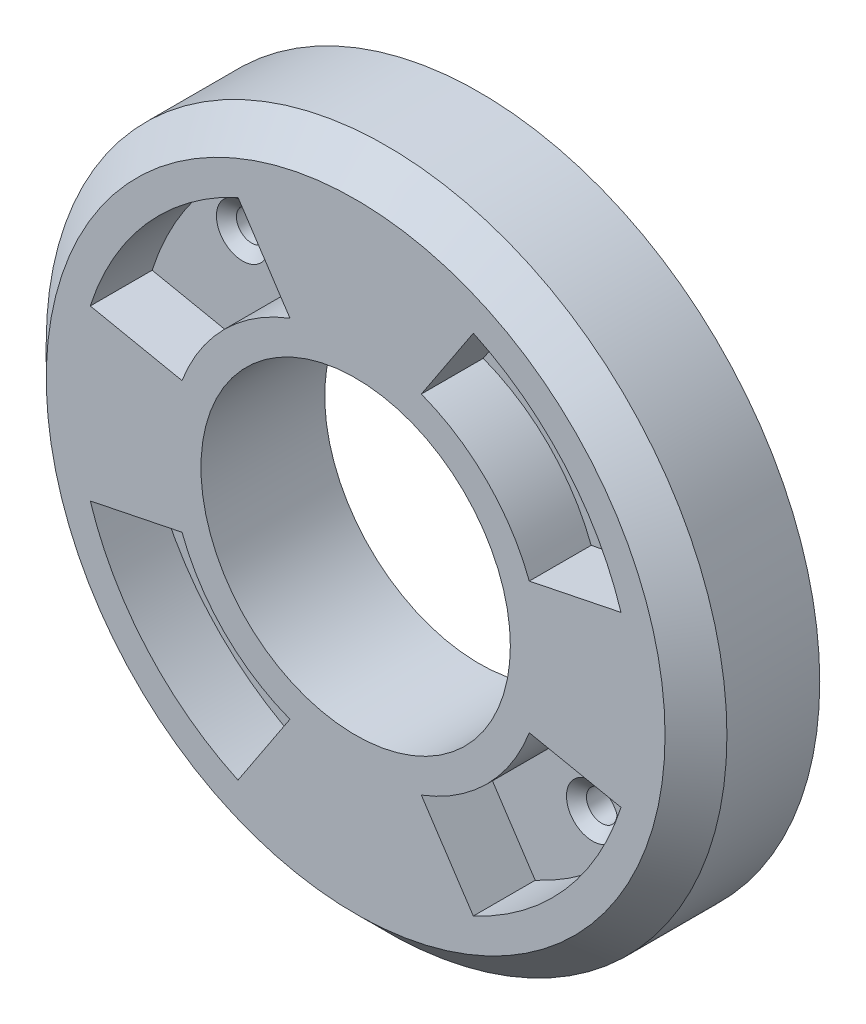
from build123d import *

# Parameters (mm, degrees)
SKETCH1_R                                         = 55
SKETCH1_R_2                                       = 25
BOSS_EXTRUDE1_DEPTH                               = 20
CUT_EXTRUDE1_DEPTH                                = 10
CHAMFER1_SIZE                                     = 5
CSK_FOR_8_FLAT_HEAD_MACHINE_SCREW_100_D           = 4.9149
CSK_FOR_8_FLAT_HEAD_MACHINE_SCREW_100_CSINK_D     = 8.4328
CSK_FOR_8_FLAT_HEAD_MACHINE_SCREW_100_CSINK_ANGLE = 100
MIRROR2_COPY_1_D                                  = 4.9149
MIRROR2_COPY_1_CSINK_D                            = 8.4328
MIRROR2_COPY_1_CSINK_ANGLE                        = 100


with BuildPart() as part:
    # Sketch1 → Boss-Extrude1 (new body)
    with BuildSketch(Plane.XY):
        Circle(SKETCH1_R)
        Circle(SKETCH1_R_2, mode=Mode.SUBTRACT)
    extrude(amount=BOSS_EXTRUDE1_DEPTH)

    # Sketch2 → Cut-Extrude1 (cut)
    with BuildSketch(Plane.XY.offset(20)):
        with BuildLine():
            Line((-10.612144625, 28.060334753), (-19.017070243, 40.784200855))
            ThreePointArc((-19.017070243, 40.784200855), (-33.794395167, 29.714287056), (-42.88237403, 13.641920597))
            Line((-42.88237403, 13.641920597), (-28.060334753, 10.612144625))
            ThreePointArc((-28.060334753, 10.612144625), (-21.213203436, 21.213203436), (-10.612144625, 28.060334753))
        make_face()
        with BuildLine():
            Line((28.060334753, 10.612144625), (42.88237403, 13.641920597))
            ThreePointArc((42.88237403, 13.641920597), (33.794395167, 29.714287056), (19.017070243, 40.784200855))
            Line((19.017070243, 40.784200855), (10.612144625, 28.060334753))
            ThreePointArc((10.612144625, 28.060334753), (21.213203436, 21.213203436), (28.060334753, 10.612144625))
        make_face()
        with BuildLine():
            Line((10.612144625, -28.060334753), (19.017070243, -40.784200855))
            ThreePointArc((19.017070243, -40.784200855), (33.794395167, -29.714287056), (42.88237403, -13.641920597))
            Line((42.88237403, -13.641920597), (28.060334753, -10.612144625))
            ThreePointArc((28.060334753, -10.612144625), (21.213203436, -21.213203436), (10.612144625, -28.060334753))
        make_face()
        with BuildLine():
            Line((-28.060334753, -10.612144625), (-42.88237403, -13.641920597))
            ThreePointArc((-42.88237403, -13.641920597), (-33.794395167, -29.714287056), (-19.017070243, -40.784200855))
            Line((-19.017070243, -40.784200855), (-10.612144625, -28.060334753))
            ThreePointArc((-10.612144625, -28.060334753), (-21.213203436, -21.213203436), (-28.060334753, -10.612144625))
        make_face()
    extrude(amount=-CUT_EXTRUDE1_DEPTH, mode=Mode.SUBTRACT)

    # Chamfer1
    chamfer1_edges = [part.edges().sort_by_distance(p)[0] for p in [
        (-55, 0, 20),
    ]]
    chamfer(chamfer1_edges, length=CHAMFER1_SIZE)

    # CSK for #8 Flat Head Machine Screw (100)1 (through all)
    with Locations(Plane(origin=(-28.284271247, 26.457513111, 10), x_dir=(1, 0, 0), z_dir=(0, 0, 1))):
        with Locations((0, 0)):
            csk_for_8_flat_head_machine_screw_100 = CounterSinkHole(CSK_FOR_8_FLAT_HEAD_MACHINE_SCREW_100_D / 2, CSK_FOR_8_FLAT_HEAD_MACHINE_SCREW_100_CSINK_D / 2, counter_sink_angle=CSK_FOR_8_FLAT_HEAD_MACHINE_SCREW_100_CSINK_ANGLE)

    # Mirror1: CSK for #8 Flat Head Machine Screw (100)1 across plane
    add(csk_for_8_flat_head_machine_screw_100.mirror(Plane(origin=(0, 0, 0), x_dir=(0, 0, 1), z_dir=(1, 0, 0))), mode=Mode.SUBTRACT)

    # Mirror2: CSK for #8 Flat Head Machine Screw (100)1 across plane
    add(csk_for_8_flat_head_machine_screw_100.mirror(Plane.ZX), mode=Mode.SUBTRACT)

    # Mirror2 copy 1 (through all)
    with Locations(Plane(origin=(28.284271247, -26.457513111, 10), x_dir=(-1, 0, 0), z_dir=(0, 0, 1))):
        with Locations((0, 0)):
            CounterSinkHole(MIRROR2_COPY_1_D / 2, MIRROR2_COPY_1_CSINK_D / 2, counter_sink_angle=MIRROR2_COPY_1_CSINK_ANGLE)


solid = part.part
